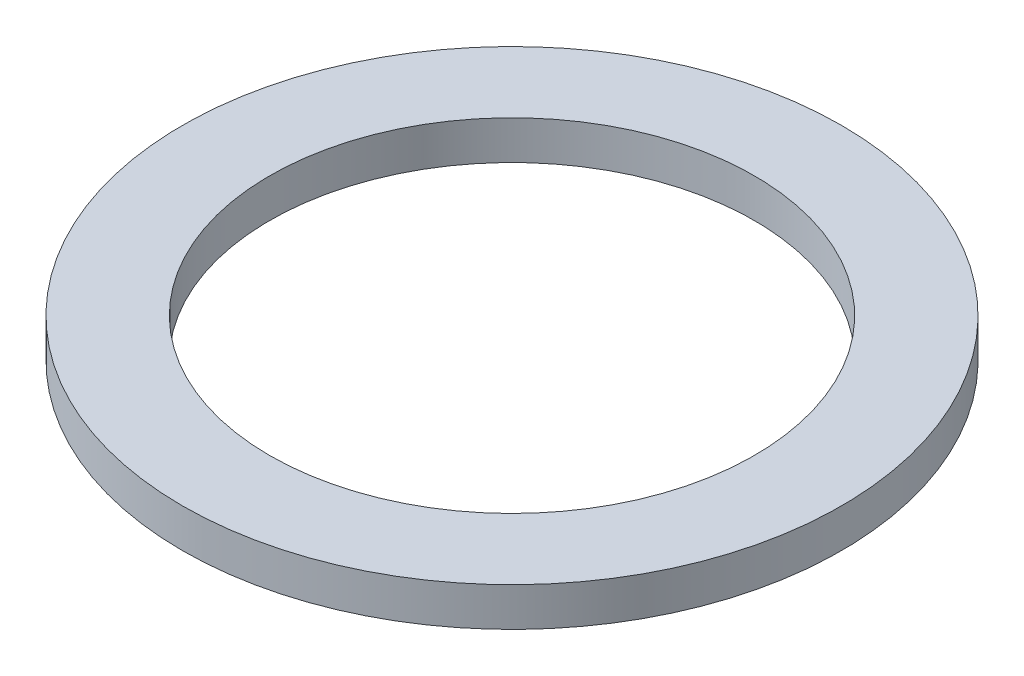
from build123d import *

# Parameters (mm, degrees)
SKETCH_1_R      = 17
SKETCH_1_R_2    = 12.5
EXTRUDE_1_DEPTH = 1


with BuildPart() as part:
    # 草图1 → 凸台-拉伸1 (new, symmetric)
    with BuildSketch(Plane(origin=(0, 0, 0), x_dir=(1, 0, 0), z_dir=(0, 1, 0))):
        with Locations(Location((0, 0, 0), (0, 0, 270))):
            Circle(SKETCH_1_R)
        with Locations(Location((0, 0, 0), (0, 0, 270))):
            Circle(SKETCH_1_R_2, mode=Mode.SUBTRACT)
    extrude(amount=EXTRUDE_1_DEPTH, both=True)


solid = part.part
